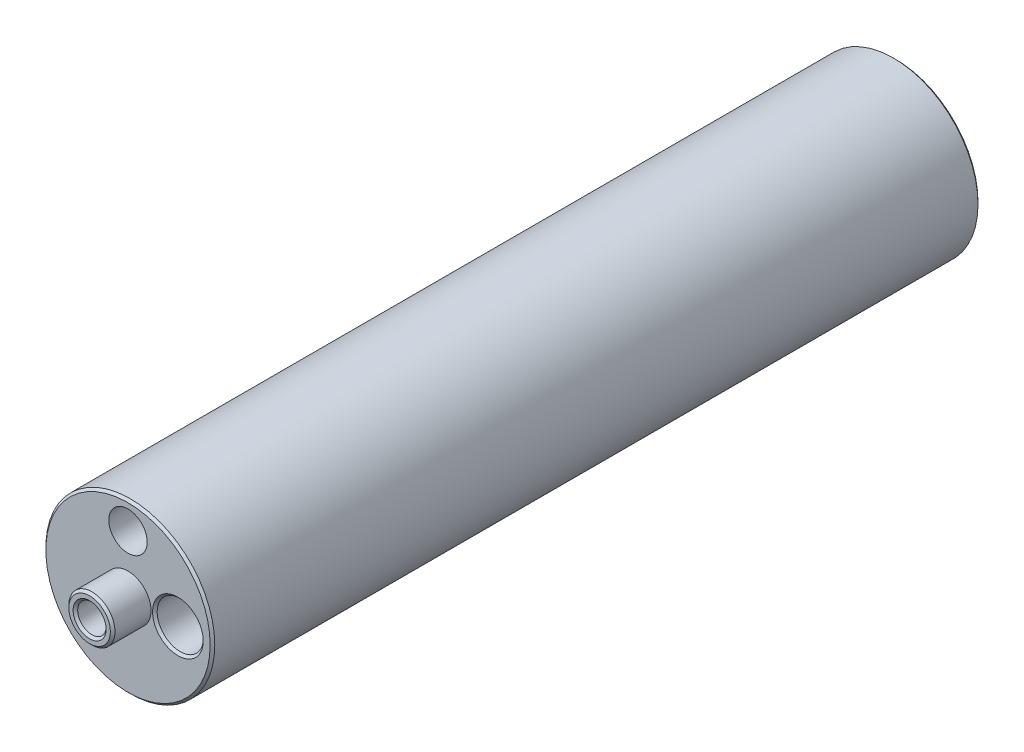
SolidWorks part; units mm, degrees
material "紫铜"
ref_plane "Front Plane" through (0, 0, 0) normal (0, 0, 1) x (1, 0, 0)
ref_plane "Top Plane" through (0, 0, 0) normal (0, 1, 0) x (1, 0, 0)
ref_plane "Right Plane" through (0, 0, 0) normal (1, 0, 0) x (0, 0, -1)
sketch "Sketch1" plane through (0, 0, 0) normal (0, 0, 1) x (1, 0, 0)
  circle A0 centre (0, 0) radius 11
  dimension "D1" = 22
extrude "Boss-Extrude1" add sketch "Sketch1" along normal blind 100
sketch "Sketch2" plane through (0, 0, 100) normal (0, 0, 1) x (1, 0, 0)
  circle A0 centre (0, 0) radius 3
  dimension "D1" = 6
extrude "Boss-Extrude2" add sketch "Sketch2" along normal blind 5
sketch "Sketch3" plane through (0, 0, 105) normal (0, 0, 1) x (1, 0, 0)
  circle A0 centre (0, 0) radius 1.85
  dimension "D1" = 3.7
extrude "Cut-Extrude1" cut sketch "Sketch3" against normal through all
sketch "Sketch4" plane through (0, 0, 100) normal (0, 0, 1) x (1, 0, 0)
  line L0 (0, 0) -> (11, 0) construction
  circle A0 centre (6.5, 0) radius 3
  circle A1 centre (0, 0) radius 11 construction
  dimension "D1" = 6
  dimension "D2" = 6.5
extrude "Cut-Extrude2" cut sketch "Sketch4" against normal through all
hole_wizard "M6 Tapped Hole1" positions "Sketch6" profile "Sketch5" tap size "M6" standard "GB"
sketch "Sketch6" plane through (0, 0, 100) normal (0, 0, 1) x (1, 0, 0)
  circle A0 centre (0, 0) radius 7.5 construction
  point P0 (0, 7.5)
  dimension "D1" = 15
sketch "Sketch5" plane through (0, 7.5, 100) normal (1, 0, 0) x (0, -1, 0)
  line L0 (0, 0) -> (0, 11.5022)
  line L1 (0, 11.5022) -> (2.5, 10)
  line L2 (2.5, 10) -> (2.5, 0)
  line L5 (2.5, 0) -> (0, 0)
  line L10 (0, 11.5022) -> (-2.5, 10) construction
  line L11 (0, -6.35) -> (0, 107.95) construction
  dimension "螺纹孔钻头直径" = 5
  dimension "螺纹孔钻头深度" = 10
  dimension "导头角度" = 118
cosmetic thread "Hole thread1" parameters "D1"=10, "D2"=6
chamfer "Chamfer1" distance 0.3 angle 45 7 edges at (9.5, 0, 100) (1.85, 0, 105) (3, 0, 105) (1.85, 0, 0) (9.5, 0, 0) (11, 0, 0) (11, 0, 100)
